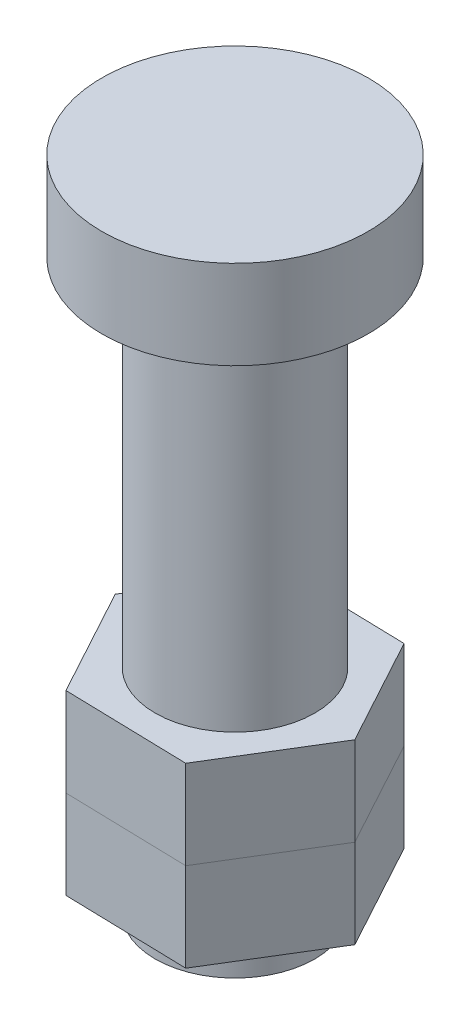
SolidWorks part; units mm, degrees
material "Q235B"
ref_plane "Front Plane" through (0, 0, 0) normal (0, 0, 1) x (1, 0, 0)
ref_plane "Top Plane" through (0, 0, 0) normal (0, 1, 0) x (1, 0, 0)
ref_plane "Right Plane" through (0, 0, 0) normal (1, 0, 0) x (0, 0, -1)
sketch "Sketch1" plane through (0, 0, 0) normal (0, 0, 1) x (1, 0, 0)
  line L0 (0, 0) -> (0, 283.9286) construction
  line L1 (0, 395.8929) -> (75, 395.8929)
  line L2 (75, 395.8929) -> (75, 345.8929)
  line L3 (75, 345.8929) -> (45, 345.8929)
  line L4 (45, 345.8929) -> (45, 25.8929)
  line L5 (45, 25.8929) -> (0, 25.8929)
  line L6 (0, 395.8929) -> (0, 25.8929)
  dimension "D1" = 320
  dimension "D2" = 90
  dimension "D3" = 150
  dimension "D4" = 50
revolve "Revolve1" add sketch "Sketch1" angle 360 about L0
ref_plane "Plane1" through (0, 145.8929, 0) normal (0, -1, 0) x (-1, 0, 0)
sketch "Sketch2" plane through (0, 145.8929, 0) normal (0, -1, 0) x (-1, 0, 0)
  line L1 (-33.101, -60.8632) -> (36.1585, -59.0979)
  line L2 (36.1585, -59.0979) -> (69.2595, 1.7653)
  line L3 (69.2595, 1.7653) -> (33.101, 60.8632)
  line L4 (33.101, 60.8632) -> (-36.1585, 59.0979)
  line L5 (-36.1585, 59.0979) -> (-69.2595, -1.7653)
  line L6 (-69.2595, -1.7653) -> (-33.101, -60.8632)
  circle A0 centre (0, 0) radius 60 construction
  circle A1 centre (0, 0) radius 45 construction
  circle A2 centre (0, 0) radius 45
  dimension "D1" = 120
extrude "Boss-Extrude1" add sketch "Sketch2" along normal blind 50 separate body
pattern_linear "LPattern1" count 2 spacing 50 along (0, -1, 0) of "Boss-Extrude1"
